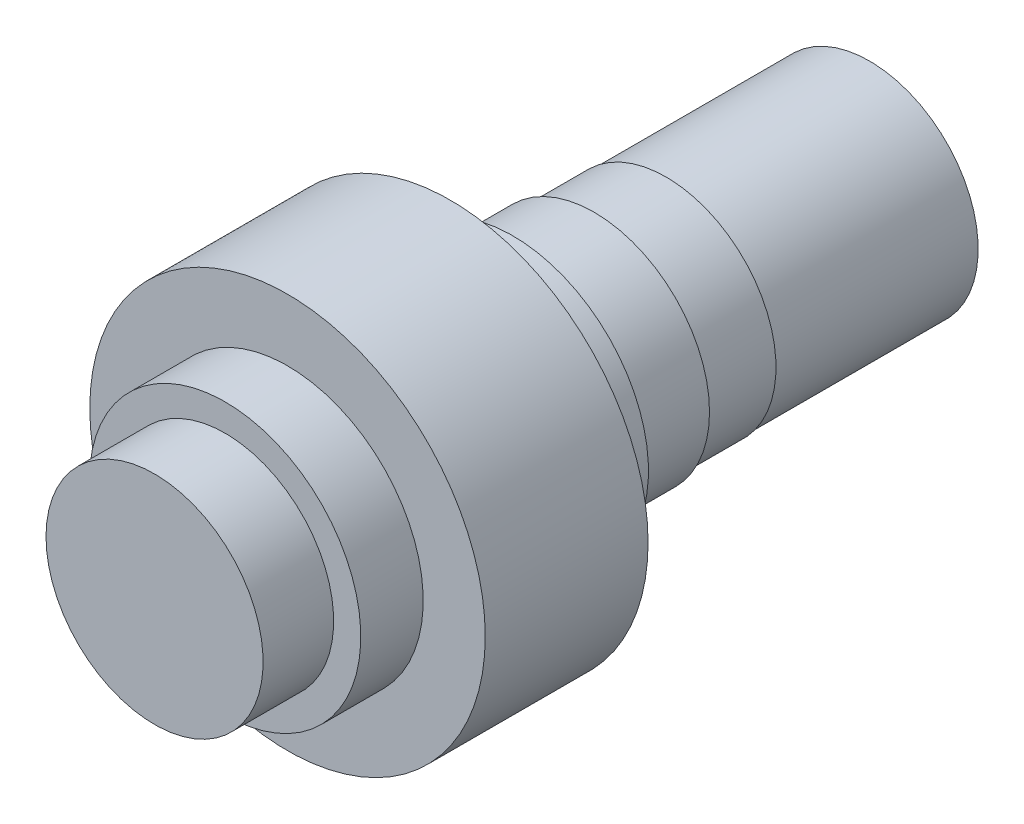
from build123d import *

# Parameters (mm, degrees)
SKETCH1_R           = 40
BOSS_EXTRUDE1_DEPTH = 26
SKETCH2_R           = 50
BOSS_EXTRUDE2_DEPTH = 23
SKETCH3_R           = 72.8615
BOSS_EXTRUDE3_DEPTH = 60
SKETCH4_R           = 50
BOSS_EXTRUDE4_DEPTH = 23
SKETCH6_R           = 42.5
BOSS_EXTRUDE5_DEPTH = 30
SKETCH7_R           = 40.5
BOSS_EXTRUDE6_DEPTH = 26.5
BOSS_EXTRUDE7_START = 75
SKETCH8_R           = 40
BOSS_EXTRUDE7_DEPTH = 75


with BuildPart() as part:
    # Sketch1 → Boss-Extrude1 (new body)
    with BuildSketch(Plane.XY):
        with Locations(Location((0, 0, 0), (0, 0, 180))):
            Circle(SKETCH1_R)
    extrude(amount=BOSS_EXTRUDE1_DEPTH)

    # Sketch2 → Boss-Extrude2 (add)
    with BuildSketch(Plane(origin=(0, 0, 0), x_dir=(-1, 0, 0), z_dir=(0, 0, -1))):
        Circle(SKETCH2_R)
    extrude(amount=BOSS_EXTRUDE2_DEPTH)

    # Sketch3 → Boss-Extrude3 (add)
    with BuildSketch(Plane(origin=(0, 0, -23), x_dir=(-1, 0, 0), z_dir=(0, 0, -1))):
        Circle(SKETCH3_R)
    extrude(amount=BOSS_EXTRUDE3_DEPTH)

    # Sketch4 → Boss-Extrude4 (add)
    with BuildSketch(Plane(origin=(0, 0, -83), x_dir=(-1, 0, 0), z_dir=(0, 0, -1))):
        Circle(SKETCH4_R)
    extrude(amount=BOSS_EXTRUDE4_DEPTH)

    # Sketch6 → Boss-Extrude5 (add)
    with BuildSketch(Plane(origin=(0, 0, -106), x_dir=(-1, 0, 0), z_dir=(0, 0, -1))):
        Circle(SKETCH6_R)
    extrude(amount=BOSS_EXTRUDE5_DEPTH)

    # Sketch7 → Boss-Extrude6 (add)
    with BuildSketch(Plane(origin=(0, 0, -136), x_dir=(-1, 0, 0), z_dir=(0, 0, -1))):
        Circle(SKETCH7_R)
    extrude(amount=BOSS_EXTRUDE6_DEPTH)

    # Sketch8 → Boss-Extrude7 (add)
    with BuildSketch(Plane(origin=(0, 0, -162.5), x_dir=(-1, 0, 0), z_dir=(0, 0, -1)).offset(BOSS_EXTRUDE7_START)):
        Circle(SKETCH8_R)
    extrude(amount=-BOSS_EXTRUDE7_DEPTH)


solid = part.part
